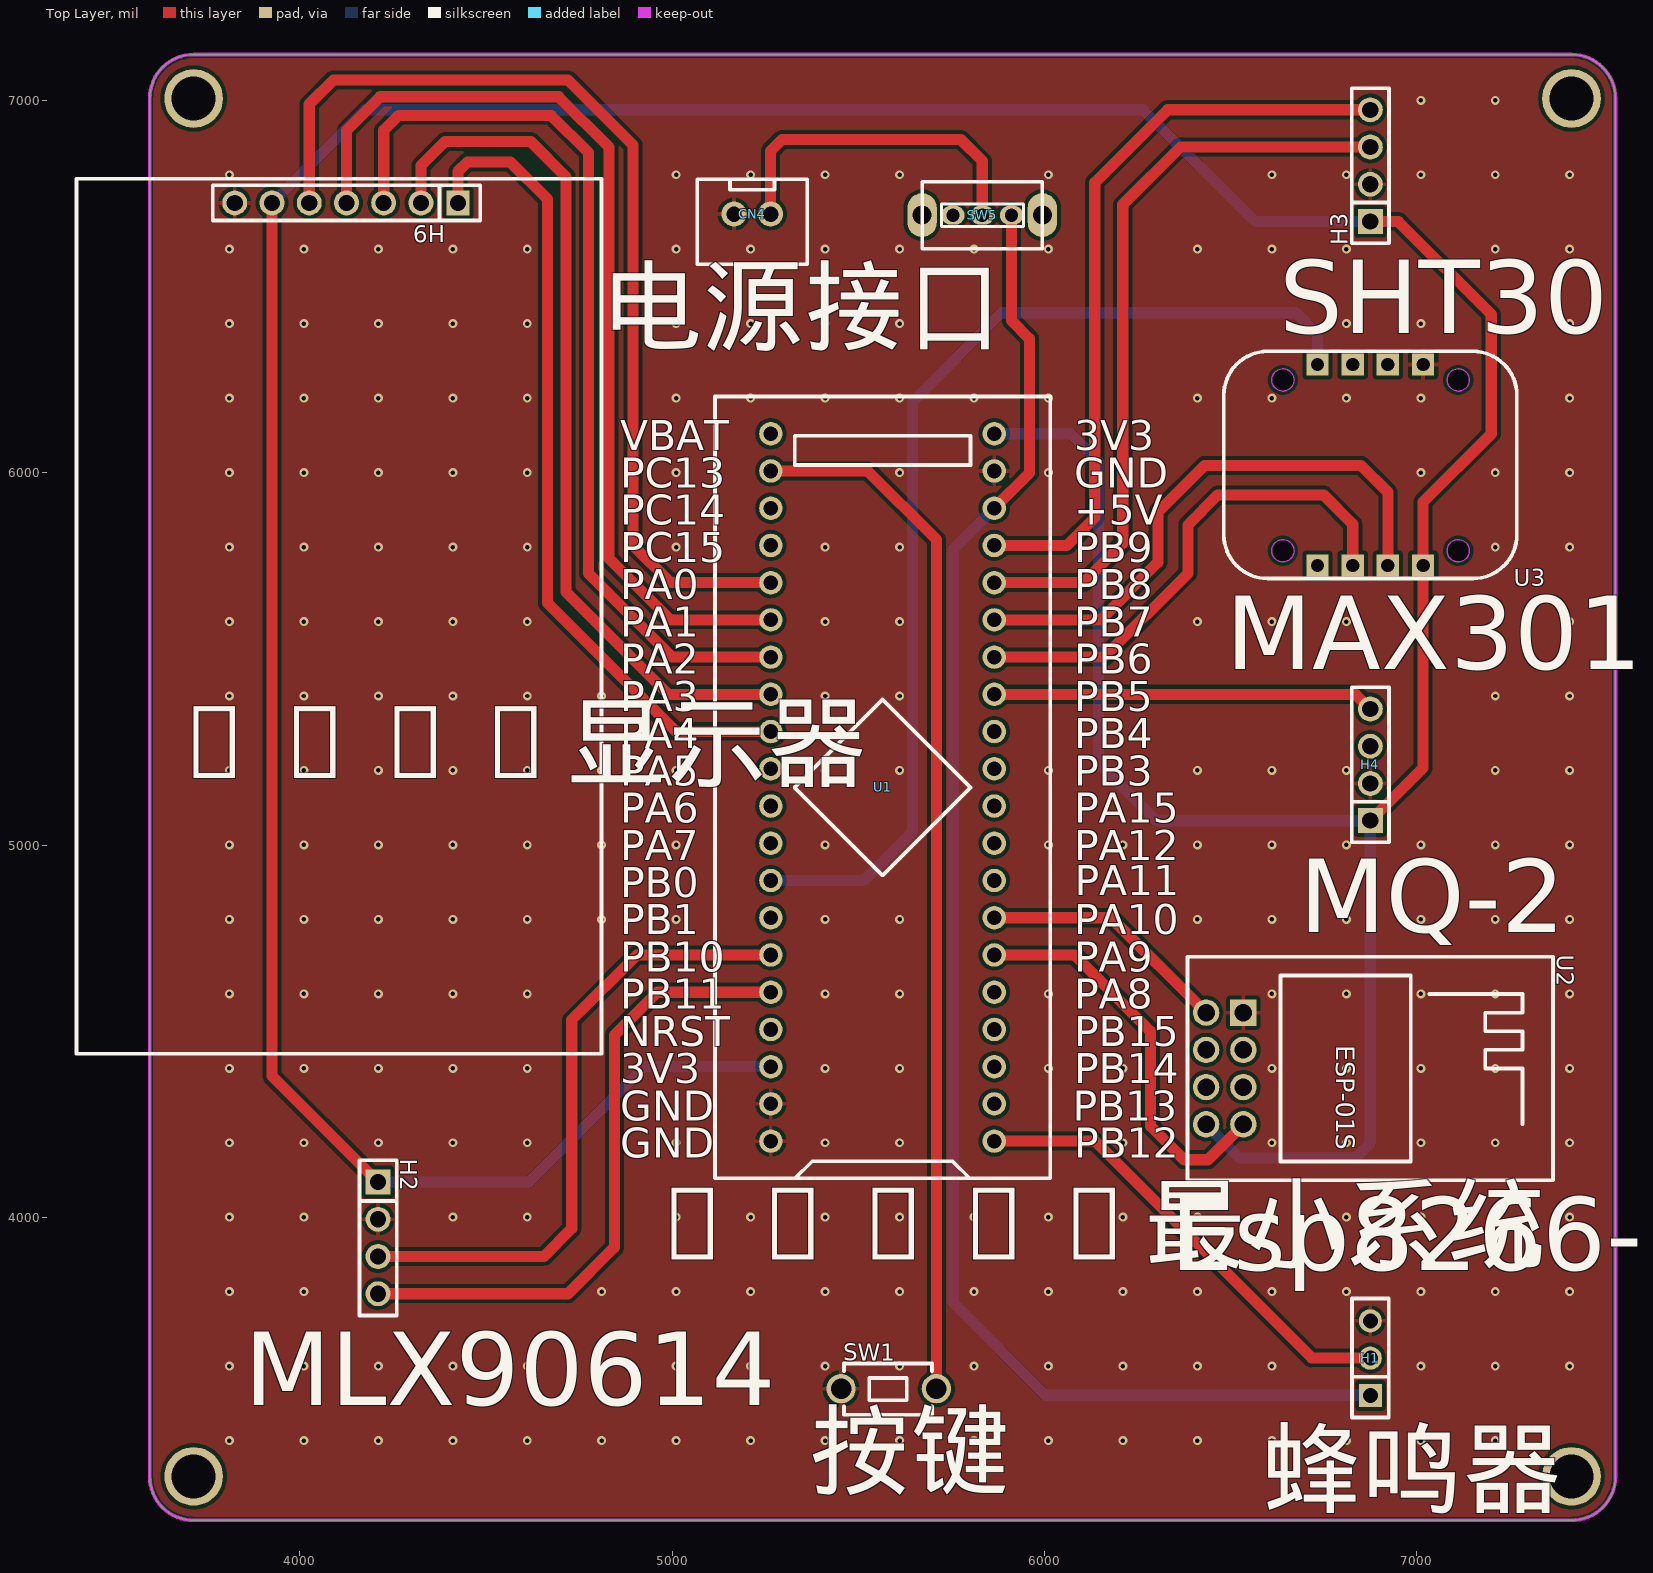
[diagram p0: Top Layer view]
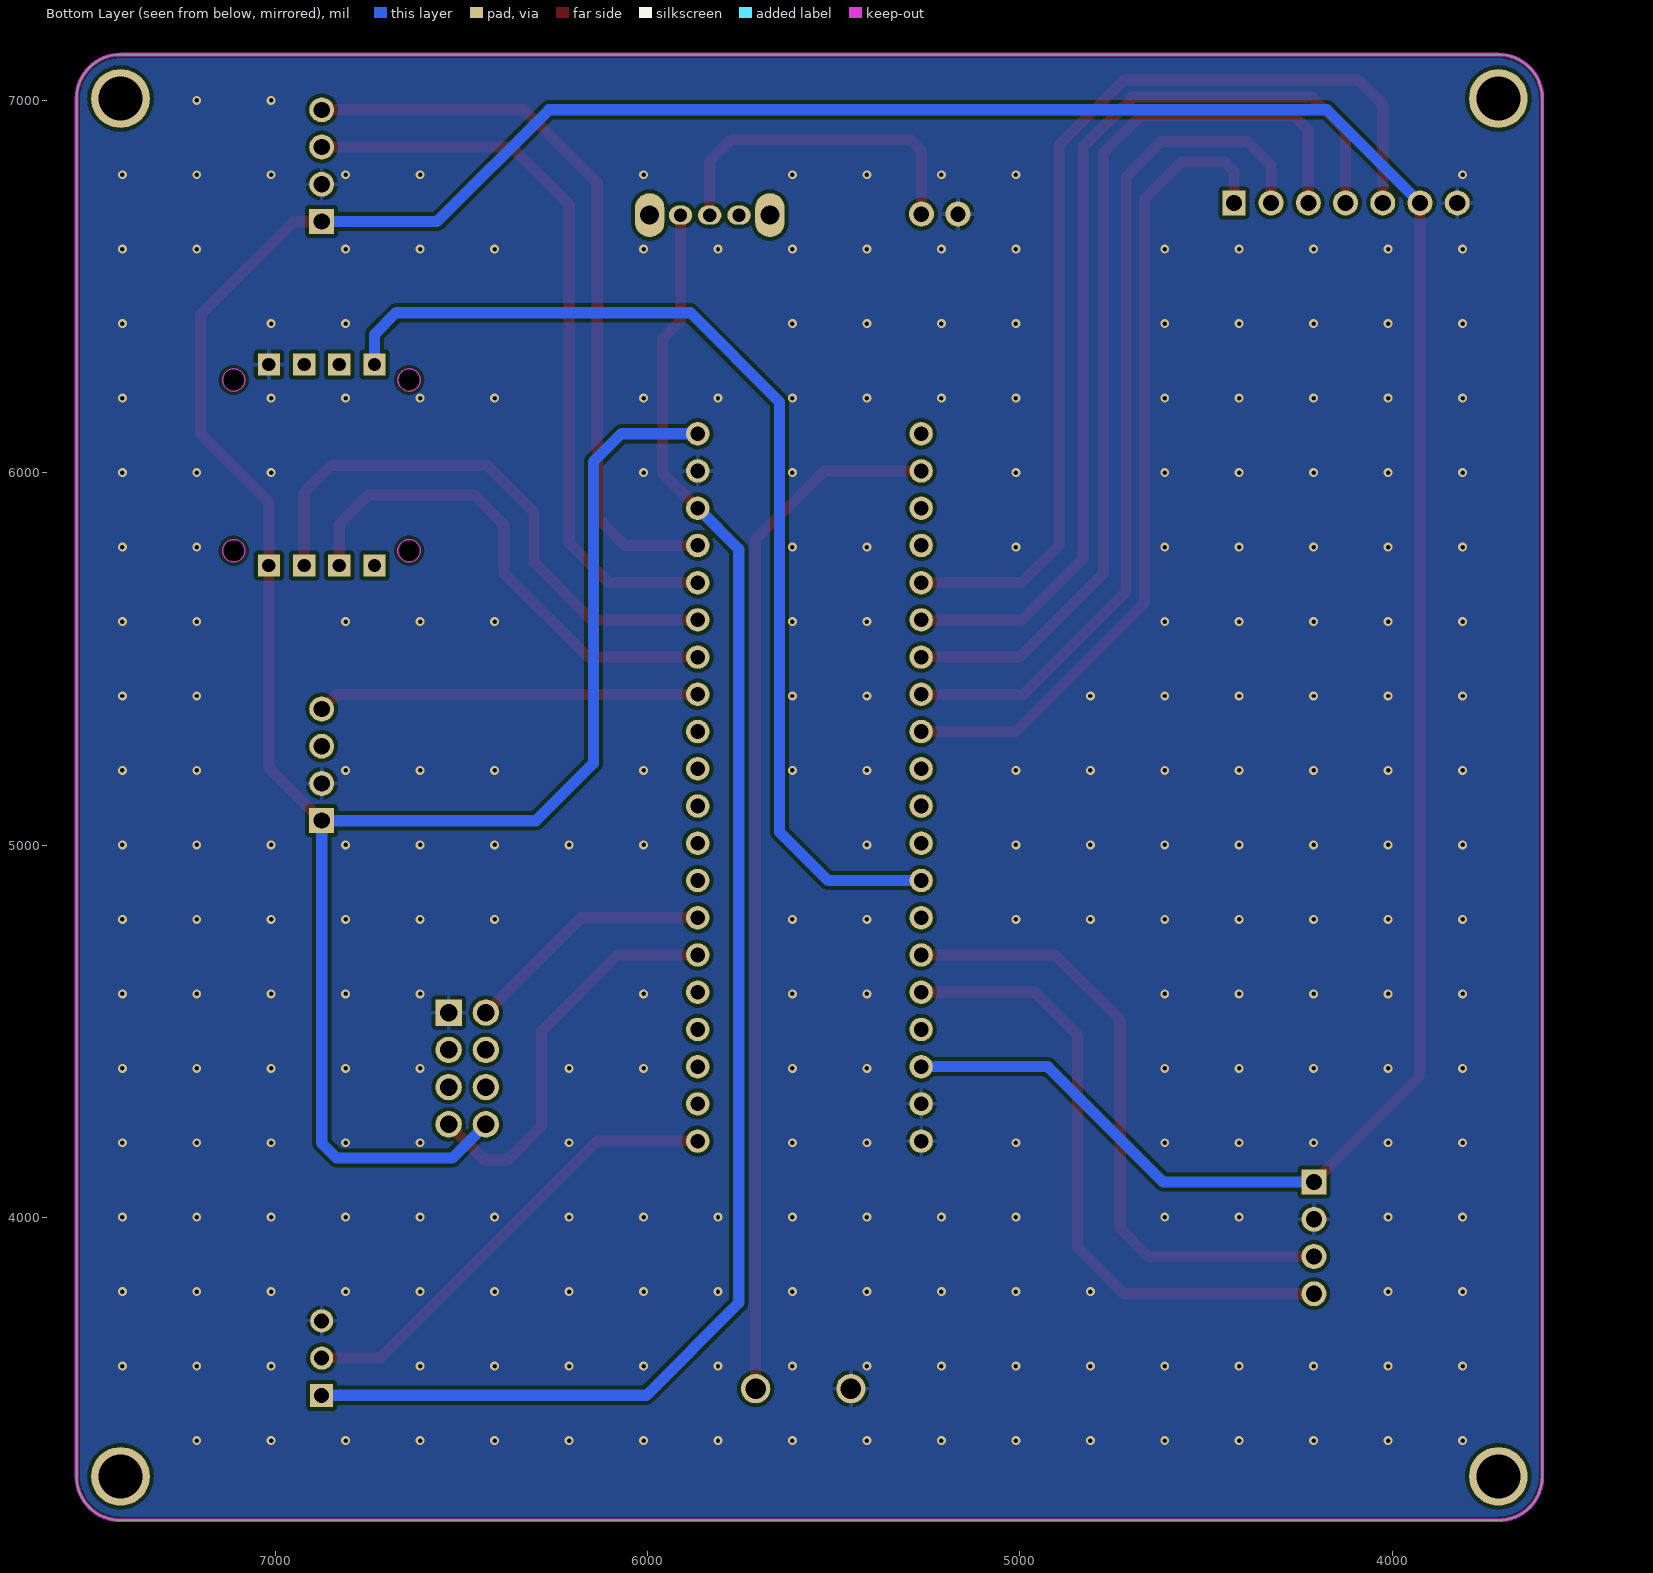
[diagram p1: Bottom Layer view, seen from below]
# Altium PCB MISC52061.pcbdoc
Units mil, origin at the board's own origin, x right, y up, seen from the top; angles counter-clockwise.
Board outline 3937.01 x 3937.01 mil, 2 copper layers (Top Layer, Bottom Layer), stack 62.206 mil thick; 11 components, 38 nets, 91 pads, 256 vias.

## Layer stack, top to bottom
Top Solder Mask Layer: solder mask 0.394, Dk 3.3
Top Layer: signal copper 1.379
Dielectric1: surface 59.449, FR4, Dk 4.5
Bottom Layer: signal copper 1.378
Bottom Solder Mask Layer: solder mask 0.394, Dk 3.3

## Board outline
3714.61,7123.5 ccw(c3714.61,7005.39) 3596.5,7005.39 3596.5,3304.61 ccw(c3714.61,3304.61) 3714.61,3186.5 7415.39,3186.5 ccw(c7415.39,3304.61) 7533.5,3304.61 7533.5,7005.39 ccw(c7415.39,7005.39) 7415.39,7123.5 3714.61,7123.5

## Design rules (kind name [scope] priority, off if disabled: settings)
BoardOutlineClearance copperThickness2oz_1 [All] p2 off: genericclearance=7.99 ignorepadtopadclearanceinfootprint=FALSE except(0: Arc-SplitContinuation Track-SplitContinuation SMDPad-SplitContinuation THPad-SplitContinuation Via-SplitContinuation Fill-SplitContinuation Region-SplitContinuation Poly-SplitContinuation Text-SplitContinuation Hole-SplitContinuation; 5.98: Arc-CutoutEdge Track-CutoutEdge SMDPad-CutoutEdge THPad-CutoutEdge Via-CutoutEdge Text-CutoutEdge; 6.9: Hole-OutlineEdge Hole-CutoutEdge; 10: Poly-OutlineEdge Poly-CutoutEdge; 11.81: Arc-OutlineEdge Track-OutlineEdge SMDPad-OutlineEdge THPad-OutlineEdge Via-OutlineEdge Fill-OutlineEdge Region-OutlineEdge Text-OutlineEdge Fill-CutoutEdge Region-CutoutEdge)
BoardOutlineClearance Plane_innerPlane_1 [All] p4 off: genericclearance=4.02 ignorepadtopadclearanceinfootprint=FALSE except(0: Arc-SplitContinuation Track-SplitContinuation SMDPad-SplitContinuation THPad-SplitContinuation Via-SplitContinuation Fill-SplitContinuation Region-SplitContinuation Poly-SplitContinuation Text-SplitContinuation Hole-SplitContinuation; 5.98: Arc-CutoutEdge Track-CutoutEdge SMDPad-CutoutEdge THPad-CutoutEdge Via-CutoutEdge Text-CutoutEdge; 6.9: Hole-OutlineEdge Hole-CutoutEdge; 10: Poly-OutlineEdge Poly-CutoutEdge; 11.81: Arc-OutlineEdge Track-OutlineEdge SMDPad-OutlineEdge THPad-OutlineEdge Via-OutlineEdge Fill-OutlineEdge Region-OutlineEdge Text-OutlineEdge Fill-CutoutEdge Region-CutoutEdge)
BoardOutlineClearance Copper_copperRegion_1 [All] p6 off: genericclearance=4.02 ignorepadtopadclearanceinfootprint=FALSE except(0: Arc-SplitContinuation Track-SplitContinuation SMDPad-SplitContinuation THPad-SplitContinuation Via-SplitContinuation Fill-SplitContinuation Region-SplitContinuation Poly-SplitContinuation Text-SplitContinuation Hole-SplitContinuation; 5.98: Arc-CutoutEdge Track-CutoutEdge SMDPad-CutoutEdge THPad-CutoutEdge Via-CutoutEdge Text-CutoutEdge; 6.9: Hole-OutlineEdge Hole-CutoutEdge; 10: Poly-OutlineEdge Poly-CutoutEdge; 11.81: Arc-OutlineEdge Track-OutlineEdge SMDPad-OutlineEdge THPad-OutlineEdge Via-OutlineEdge Fill-OutlineEdge Region-OutlineEdge Text-OutlineEdge Fill-CutoutEdge Region-CutoutEdge)
BoardOutlineClearance Copper_copperRegion_copperThickness1oz_1 [All] p8 off: genericclearance=4.02 ignorepadtopadclearanceinfootprint=FALSE except(0: Arc-SplitContinuation Track-SplitContinuation SMDPad-SplitContinuation THPad-SplitContinuation Via-SplitContinuation Fill-SplitContinuation Region-SplitContinuation Poly-SplitContinuation Text-SplitContinuation Hole-SplitContinuation; 5.98: Arc-CutoutEdge Track-CutoutEdge SMDPad-CutoutEdge THPad-CutoutEdge Via-CutoutEdge Text-CutoutEdge; 6.9: Hole-OutlineEdge Hole-CutoutEdge; 10: Poly-OutlineEdge Poly-CutoutEdge; 11.81: Arc-OutlineEdge Track-OutlineEdge SMDPad-OutlineEdge THPad-OutlineEdge Via-OutlineEdge Fill-OutlineEdge Region-OutlineEdge Text-OutlineEdge Fill-CutoutEdge Region-CutoutEdge)
BoardOutlineClearance Copper_copperRegion_Copper_copperRegion_1 [All] p10 off: genericclearance=4.02 ignorepadtopadclearanceinfootprint=FALSE except(0: Arc-SplitContinuation Track-SplitContinuation SMDPad-SplitContinuation THPad-SplitContinuation Via-SplitContinuation Fill-SplitContinuation Region-SplitContinuation Poly-SplitContinuation Text-SplitContinuation Hole-SplitContinuation; 5.98: Arc-CutoutEdge Track-CutoutEdge SMDPad-CutoutEdge THPad-CutoutEdge Via-CutoutEdge Text-CutoutEdge; 6.9: Hole-OutlineEdge Hole-CutoutEdge; 10: Poly-OutlineEdge Poly-CutoutEdge; 11.81: Arc-OutlineEdge Track-OutlineEdge SMDPad-OutlineEdge THPad-OutlineEdge Via-OutlineEdge Fill-OutlineEdge Region-OutlineEdge Text-OutlineEdge Fill-CutoutEdge Region-CutoutEdge)
BoardOutlineClearance copperThickness1oz_1 [All] p12: genericclearance=4.02 ignorepadtopadclearanceinfootprint=FALSE except(0: Arc-SplitContinuation Track-SplitContinuation SMDPad-SplitContinuation THPad-SplitContinuation Via-SplitContinuation Fill-SplitContinuation Region-SplitContinuation Poly-SplitContinuation Text-SplitContinuation Hole-SplitContinuation; 5.98: Arc-CutoutEdge Track-CutoutEdge SMDPad-CutoutEdge THPad-CutoutEdge Via-CutoutEdge Text-CutoutEdge; 6.9: Hole-OutlineEdge Hole-CutoutEdge; 10: Poly-OutlineEdge Poly-CutoutEdge; 11.81: Arc-OutlineEdge Track-OutlineEdge SMDPad-OutlineEdge THPad-OutlineEdge Via-OutlineEdge Fill-OutlineEdge Region-OutlineEdge Text-OutlineEdge Fill-CutoutEdge Region-CutoutEdge)
Clearance copperThickness2oz [All] p1 off: gap=7.99 ignorepadtopadclearanceinfootprint=FALSE except(5.98: SMDPad-Track SMDPad-SMDPad THPad-Track SMDPad-THPad THPad-THPad Track-Via SMDPad-Via THPad-Via Via-Via Fill-SMDPad Region-SMDPad Fill-THPad Region-THPad Fill-Via Region-Via Fill-Fill Fill-Region Region-Region Arc-Track Arc-SMDPad Arc-THPad Arc-Via Fill-Arc Region-Arc Arc-Arc Text-Track SMDPad-Text Text-THPad Text-Via Fill-Text Region-Text Arc-Text Text-Text; 6.9: Hole-Track Hole-SMDPad Hole-THPad Hole-Via Fill-Hole Region-Hole Hole-Arc Hole-Text; 10: Poly-Track Poly-SMDPad Poly-THPad Poly-Via Poly-Fill Poly-Region Poly-Poly Poly-Arc Poly-Text Poly-Hole; 11.81: Fill-Track Region-Track)
Clearance Plane_innerPlane [All] p3 off: gap=4.02 ignorepadtopadclearanceinfootprint=FALSE except(5.98: SMDPad-Track SMDPad-SMDPad THPad-Track SMDPad-THPad THPad-THPad Track-Via SMDPad-Via THPad-Via Via-Via Fill-SMDPad Region-SMDPad Fill-THPad Region-THPad Fill-Via Region-Via Fill-Fill Fill-Region Region-Region Arc-Track Arc-SMDPad Arc-THPad Arc-Via Fill-Arc Region-Arc Arc-Arc Text-Track SMDPad-Text Text-THPad Text-Via Fill-Text Region-Text Arc-Text Text-Text; 6.9: Hole-Track Hole-SMDPad Hole-THPad Hole-Via Fill-Hole Region-Hole Hole-Arc Hole-Text; 10: Poly-Track Poly-SMDPad Poly-THPad Poly-Via Poly-Fill Poly-Region Poly-Poly Poly-Arc Poly-Text Poly-Hole; 11.81: Fill-Track Region-Track)
Clearance Copper_copperRegion [All] p5 off: gap=4.02 ignorepadtopadclearanceinfootprint=FALSE except(5.98: SMDPad-Track SMDPad-SMDPad THPad-Track SMDPad-THPad THPad-THPad Track-Via SMDPad-Via THPad-Via Via-Via Fill-SMDPad Region-SMDPad Fill-THPad Region-THPad Fill-Via Region-Via Fill-Fill Fill-Region Region-Region Arc-Track Arc-SMDPad Arc-THPad Arc-Via Fill-Arc Region-Arc Arc-Arc Text-Track SMDPad-Text Text-THPad Text-Via Fill-Text Region-Text Arc-Text Text-Text; 6.9: Hole-Track Hole-SMDPad Hole-THPad Hole-Via Fill-Hole Region-Hole Hole-Arc Hole-Text; 10: Poly-Track Poly-SMDPad Poly-THPad Poly-Via Poly-Fill Poly-Region Poly-Poly Poly-Arc Poly-Text Poly-Hole; 11.81: Fill-Track Region-Track)
Clearance Copper_copperRegion_copperThickness1oz [All] p7 off: gap=4.02 ignorepadtopadclearanceinfootprint=FALSE except(5.98: SMDPad-Track SMDPad-SMDPad THPad-Track SMDPad-THPad THPad-THPad Track-Via SMDPad-Via THPad-Via Via-Via Fill-SMDPad Region-SMDPad Fill-THPad Region-THPad Fill-Via Region-Via Fill-Fill Fill-Region Region-Region Arc-Track Arc-SMDPad Arc-THPad Arc-Via Fill-Arc Region-Arc Arc-Arc Text-Track SMDPad-Text Text-THPad Text-Via Fill-Text Region-Text Arc-Text Text-Text; 6.9: Hole-Track Hole-SMDPad Hole-THPad Hole-Via Fill-Hole Region-Hole Hole-Arc Hole-Text; 10: Poly-Track Poly-SMDPad Poly-THPad Poly-Via Poly-Fill Poly-Region Poly-Poly Poly-Arc Poly-Text Poly-Hole; 11.81: Fill-Track Region-Track)
Clearance Copper_copperRegion_Copper_copperRegion [All] p9 off: gap=4.02 ignorepadtopadclearanceinfootprint=FALSE except(5.98: SMDPad-Track SMDPad-SMDPad THPad-Track SMDPad-THPad THPad-THPad Track-Via SMDPad-Via THPad-Via Via-Via Fill-SMDPad Region-SMDPad Fill-THPad Region-THPad Fill-Via Region-Via Fill-Fill Fill-Region Region-Region Arc-Track Arc-SMDPad Arc-THPad Arc-Via Fill-Arc Region-Arc Arc-Arc Text-Track SMDPad-Text Text-THPad Text-Via Fill-Text Region-Text Arc-Text Text-Text; 6.9: Hole-Track Hole-SMDPad Hole-THPad Hole-Via Fill-Hole Region-Hole Hole-Arc Hole-Text; 10: Poly-Track Poly-SMDPad Poly-THPad Poly-Via Poly-Fill Poly-Region Poly-Poly Poly-Arc Poly-Text Poly-Hole; 11.81: Fill-Track Region-Track)
Clearance copperThickness1oz [All] p11: gap=4.02 ignorepadtopadclearanceinfootprint=FALSE except(5.98: SMDPad-Track SMDPad-SMDPad THPad-Track SMDPad-THPad THPad-THPad Track-Via SMDPad-Via THPad-Via Via-Via Fill-SMDPad Region-SMDPad Fill-THPad Region-THPad Fill-Via Region-Via Fill-Fill Fill-Region Region-Region Arc-Track Arc-SMDPad Arc-THPad Arc-Via Fill-Arc Region-Arc Arc-Arc Text-Track SMDPad-Text Text-THPad Text-Via Fill-Text Region-Text Arc-Text Text-Text; 6.9: Hole-Track Hole-SMDPad Hole-THPad Hole-Via Fill-Hole Region-Hole Hole-Arc Hole-Text; 10: Poly-Track Poly-SMDPad Poly-THPad Poly-Via Poly-Fill Poly-Region Poly-Poly Poly-Arc Poly-Text Poly-Hole; 11.81: Fill-Track Region-Track)
DiffPairsRouting differentialPair [All] p1: maxlimit=6 minlimit=6 mostfreqgap=6 toplayer_minwidth=5 toplayer_prefwidth=10 toplayer_maxwidth=100 toplayer_mingap=6 toplayer_prefgap=6 toplayer_maxgap=6 bottomlayer_minwidth=5 bottomlayer_prefwidth=10 bottomlayer_maxwidth=100 bottomlayer_mingap=6 bottomlayer_prefgap=6 bottomlayer_maxgap=6 maxuncoupledlength=10
HoleToHoleClearance otherClearance [All] p1: gap=11.81 allowstackedmicrovias=TRUE
Length netLength [All] p1: minlimit=0 maxlimit=0
PasteMaskExpansion pasteMaskExpansion [All] p1: expansion=0
PlaneConnect innerPlane [All] p1: planeconnectstyle=Relief reliefexpansion=20 reliefentries=4 reliefconductorwidth=10 reliefairgap=10
PolygonConnect copperRegion_copperThickness1oz [All] p1 off: connectstyle=Relief reliefconductorwidth=10 reliefentries=4 polygonreliefangle="90 Angle" airgapwidth=10 via.connectstyle=Relief via.reliefconductorwidth=10 via.reliefentries=4 via.polygonreliefangle="90 Angle" via.airgapwidth=10
PolygonConnect copperRegion_Copper_copperRegion [All] p2 off: connectstyle=Relief reliefconductorwidth=10 reliefentries=4 polygonreliefangle="90 Angle" airgapwidth=10 via.connectstyle=Relief via.reliefconductorwidth=10 via.reliefentries=4 via.polygonreliefangle="90 Angle" via.airgapwidth=10
PolygonConnect copperRegion [All] p3: connectstyle=Relief reliefconductorwidth=10 reliefentries=4 polygonreliefangle="90 Angle" airgapwidth=10 via.connectstyle=Relief via.reliefconductorwidth=10 via.reliefentries=4 via.polygonreliefangle="90 Angle" via.airgapwidth=10
RoutingVias viaSize [All] p1: holewidth=12.01 width=24.02 viastyle="Through Hole" minholewidth=11.81 minwidth=19.68 maxholewidth=248.03 maxwidth=393.7
SolderMaskExpansion solderMaskExpansion [IsVia] p1: expansion=-1000 istentingtop=TRUE
SolderMaskExpansion solderMaskExpansion [All] p2: expansion=2 istentingtop=FALSE
Width copperThickness2oz_2 [All] p1 off: maxlimit=100 minlimit=8 preferedwidth=10
Width copperThickness1oz_2 [All] p2: maxlimit=100 minlimit=5 preferedwidth=10

## Components (designator, comment, footprint, x,y, rotation, side; value= is the part's Value field where it differs from the comment)
CN4 "XH2.54*2P_直插" CONN-TH_2P-P2.50-XH2.54-2P 5215,6695 r0 top
H1 "" HDR-TH_3P-P2.54-V-F 6875,3622.19 r90 top
H2 "" HDR-TH_4P-P2.54-V-F 4210,3945 r270 top
H3 "" HDR-TH_4P-P2.54-V-F 6875,6825 r90 top
H4 "" HDR-TH_4P-P2.54-V-F 6875,5215.69 r90 top
H9 "" HDR-TH_7P-P2.54-V-F 4125,6725 r180 top
SW1 "" Key_TH_3.5x6x4.3 5575,3540 r0 top
SW5 "" 拨动开关 5837.9,6692.05 r180 top
U1 "STM32F103C8T6-Card" CONN-TH_L53.3-W22.9_STM32F103C8T6-CARD 5565,5155 r90 top
U2 "ESP-01S" WIFIM-TH_ESP-01S 6484,4400.1 r270 top
U3 "MAX30102" MAX30102 7268.7,5715.97 r180 top

## Footprints (in the part's own frame and the unit in brackets; to place one, negate y for a bottom-side part, rotate by r counter-clockwise, add the part's x,y. Pads: shape width x height; smd on the part's side, far side on the other; paste and mask are expansions set on the pad)
CONN-TH_2P-P2.50-XH2.54-2P [mm]
  round 1.7 hole 1.05 paste+0 mask+0.05: 1(1.25,0) 2(-1.25,0)
  silkscreen extent -3.75,-3.42 3.75,2.37
CONN-TH_L53.3-W22.9_STM32F103C8T6-CARD [mm]
  round 1.6 hole 1: 1(-24.13,-7.62) 2(-21.59,-7.62) 3(-19.05,-7.62) 4(-16.51,-7.62) 5(-13.97,-7.62) 6(-11.43,-7.62) 7(-8.89,-7.62) 8(-6.35,-7.62) 9(-3.81,-7.62) 10(-1.27,-7.62) 11(1.27,-7.62) 12(3.81,-7.62) 13(6.35,-7.62) 14(8.89,-7.62) 15(11.43,-7.62) 16(13.97,-7.62) 17(16.51,-7.62) 18(19.05,-7.62) 19(21.59,-7.62) 20(24.13,-7.62) 21(24.13,7.62) 22(21.59,7.62) 23(19.05,7.62) 24(16.51,7.62) 25(13.97,7.62) 26(11.43,7.62) 27(8.89,7.62) 28(6.35,7.62) 29(3.81,7.62) 30(1.27,7.62) 31(-1.27,7.62) 32(-3.81,7.62) 33(-6.35,7.62) 34(-8.89,7.62) 35(-11.43,7.62) 36(-13.97,7.62) 37(-16.51,7.62) 38(-19.05,7.62) 39(-21.59,7.62) 40(-24.13,7.62)
  silkscreen extent -26.67,-11.43 26.67,11.43
HDR-TH_3P-P2.54-V-F [mil]
  rect 62x62 hole 40.16: 1(-100,0)
  round 62 hole 40.16: 2(0,0) 3(100,0)
  silkscreen extent -160,-49 160,49
HDR-TH_4P-P2.54-V-F [mm]
  rect 1.7x1.7 hole 1.1: 1(-3.81,0)
  round 1.7 hole 1.1: 2(-1.27,0) 3(1.27,0) 4(3.81,0)
  silkscreen extent -5.29,-1.27 5.29,1.27
HDR-TH_7P-P2.54-V-F [mm]
  rect 1.575x1.7 hole 1.1: 1(-7.62,0)
  round 1.7 hole 1.1: 2(-5.08,0) 3(-2.54,0) 4(0,0) 5(2.54,0) 6(5.08,0) 7(7.62,0)
  silkscreen extent -9.13,-1.2 9.13,1.2
Key_TH_3.5x6x4.3 [mil]
  round 78.7 hole 55.1 paste+0 mask+2: A(-121.44,0) B(134.46,0)
  silkscreen extent -114,-70 123,68
MAX30102 [mil]
  rect 60x60 hole 36: 1(251.97,-35) 2(346.46,-35) 3(440.94,-35) 4(535.43,-35) 5(251.97,-575) 6(346.46,-575) 7(440.94,-575) 8(535.43,-575)
  Board Outline Layer circle w0.1: c157.48,-74.8 r30
  Board Outline Layer circle w0.1: c157.48,-533.46 r30
  Board Outline Layer circle w0.1: c628.5,-74.8 r30
  Board Outline Layer circle w0.1: c628.5,-533.46 r30
  Board Outline Layer region: 127.48,-74.8 130.45,-61.79 138.78,-51.35 150.8,-45.56 164.16,-45.56 176.18,-51.35 184.51,-61.79 187.48,-74.8 187.48,-74.8 184.51,-87.82 176.18,-98.26 164.16,-104.05 150.8,-104.05 138.78,-98.26 130.45,-87.82 127.48,-74.8
  Board Outline Layer region: 127.48,-74.8 127.85,-70.11 128.95,-65.53 130.75,-61.18 133.21,-57.17 136.27,-53.59 139.85,-50.53 143.86,-48.07 148.21,-46.27 152.79,-45.17 157.48,-44.8 162.17,-45.17 166.75,-46.27 171.1,-48.07 175.11,-50.53 178.69,-53.59 181.75,-57.17 184.21,-61.18 186.01,-65.53 187.11,-70.11 187.48,-74.8 187.11,-79.5 186.01,-84.07 184.21,-88.42 181.75,-92.44 178.69,-96.02 175.11,-99.07 171.1,-101.53 166.75,-103.33 162.17,-104.43 157.48,-104.8 152.79,-104.43 148.21,-103.33 143.86,-101.53 139.85,-99.07 136.27,-96.02 133.21,-92.44 130.75,-88.42 128.95,-84.07 127.85,-79.5
  Board Outline Layer region: 127.48,-533.46 130.45,-520.45 138.78,-510.01 150.8,-504.22 164.16,-504.22 176.18,-510.01 184.51,-520.45 187.48,-533.46 187.48,-533.46 184.51,-546.48 176.18,-556.92 164.16,-562.71 150.8,-562.71 138.78,-556.92 130.45,-546.48 127.48,-533.46
  Board Outline Layer region: 127.48,-533.46 127.85,-528.77 128.95,-524.19 130.75,-519.84 133.21,-515.83 136.27,-512.25 139.85,-509.19 143.86,-506.73 148.21,-504.93 152.79,-503.83 157.48,-503.46 162.17,-503.83 166.75,-504.93 171.1,-506.73 175.11,-509.19 178.69,-512.25 181.75,-515.83 184.21,-519.84 186.01,-524.19 187.11,-528.77 187.48,-533.46 187.11,-538.16 186.01,-542.74 184.21,-547.08 181.75,-551.1 178.69,-554.68 175.11,-557.74 171.1,-560.19 166.75,-562 162.17,-563.1 157.48,-563.46 152.79,-563.1 148.21,-562 143.86,-560.19 139.85,-557.74 136.27,-554.68 133.21,-551.1 130.75,-547.08 128.95,-542.74 127.85,-538.16
  Board Outline Layer region: 598.5,-74.8 601.47,-61.79 609.8,-51.35 621.83,-45.56 635.18,-45.56 647.21,-51.35 655.53,-61.79 658.5,-74.8 658.5,-74.8 655.53,-87.82 647.21,-98.26 635.18,-104.05 621.83,-104.05 609.8,-98.26 601.47,-87.82 598.5,-74.8
  Board Outline Layer region: 598.5,-74.8 598.87,-70.11 599.97,-65.53 601.77,-61.18 604.23,-57.17 607.29,-53.59 610.87,-50.53 614.88,-48.07 619.23,-46.27 623.81,-45.17 628.5,-44.8 633.2,-45.17 637.77,-46.27 642.12,-48.07 646.14,-50.53 649.72,-53.59 652.77,-57.17 655.23,-61.18 657.04,-65.53 658.13,-70.11 658.5,-74.8 658.13,-79.5 657.04,-84.07 655.23,-88.42 652.77,-92.44 649.72,-96.02 646.14,-99.07 642.12,-101.53 637.77,-103.33 633.2,-104.43 628.5,-104.8 623.81,-104.43 619.23,-103.33 614.88,-101.53 610.87,-99.07 607.29,-96.02 604.23,-92.44 601.77,-88.42 599.97,-84.07 598.87,-79.5
  Board Outline Layer region: 598.5,-533.46 601.47,-520.45 609.8,-510.01 621.83,-504.22 635.18,-504.22 647.21,-510.01 655.53,-520.45 658.5,-533.46 658.5,-533.46 655.53,-546.48 647.21,-556.92 635.18,-562.71 621.83,-562.71 609.8,-556.92 601.47,-546.48 598.5,-533.46
  Board Outline Layer region: 598.5,-533.46 598.87,-528.77 599.97,-524.19 601.77,-519.84 604.23,-515.83 607.29,-512.25 610.87,-509.19 614.88,-506.73 619.23,-504.93 623.81,-503.83 628.5,-503.46 633.2,-503.83 637.77,-504.93 642.12,-506.73 646.14,-509.19 649.72,-512.25 652.77,-515.83 655.23,-519.84 657.04,-524.19 658.13,-528.77 658.5,-533.46 658.13,-538.16 657.04,-542.74 655.23,-547.08 652.77,-551.1 649.72,-554.68 646.14,-557.74 642.12,-560.19 637.77,-562 633.2,-563.1 628.5,-563.46 623.81,-563.1 619.23,-562 614.88,-560.19 610.87,-557.74 607.29,-554.68 604.23,-551.1 601.77,-547.08 599.97,-542.74 598.87,-538.16
  Multi-Layer board cut-out: 127.48,-74.8 130.45,-61.79 138.78,-51.35 150.8,-45.56 164.16,-45.56 176.18,-51.35 184.51,-61.79 187.48,-74.8 187.48,-74.8 184.51,-87.82 176.18,-98.26 164.16,-104.05 150.8,-104.05 138.78,-98.26 130.45,-87.82 127.48,-74.8
  Multi-Layer board cut-out: 127.48,-533.46 130.45,-520.45 138.78,-510.01 150.8,-504.22 164.16,-504.22 176.18,-510.01 184.51,-520.45 187.48,-533.46 187.48,-533.46 184.51,-546.48 176.18,-556.92 164.16,-562.71 150.8,-562.71 138.78,-556.92 130.45,-546.48 127.48,-533.46
  Multi-Layer board cut-out: 598.5,-74.8 601.47,-61.79 609.8,-51.35 621.83,-45.56 635.18,-45.56 647.21,-51.35 655.53,-61.79 658.5,-74.8 658.5,-74.8 655.53,-87.82 647.21,-98.26 635.18,-104.05 621.83,-104.05 609.8,-98.26 601.47,-87.82 598.5,-74.8
  Multi-Layer board cut-out: 598.5,-533.46 601.47,-520.45 609.8,-510.01 621.83,-504.22 635.18,-504.22 647.21,-510.01 655.53,-520.45 658.5,-533.46 658.5,-533.46 655.53,-546.48 647.21,-556.92 635.18,-562.71 621.83,-562.71 609.8,-556.92 601.47,-546.48 598.5,-533.46
  silkscreen extent 0,-610 787,0
WIFIM-TH_ESP-01S [mm]
  rect 1.8x1.8 hole 1.2: 1(-3.81,1.27)
  round 1.8 hole 1.2: 2(-1.27,1.27) 3(1.27,1.27) 4(3.81,1.27) 5(3.81,-1.27) 6(1.27,-1.27) 7(-1.27,-1.27) 8(-3.81,-1.27)
  silkscreen extent -7.62,-2.54 7.62,22.4
拨动开关 [mil]
  oval 63x51.2 hole 35.4 paste+0 mask+2: 1(-73.4,0) 2(5,0) 3(84,0)
  oval 78.7x118.1 hole 51.2 paste+0 mask+2: 4(166.7,0) 5(-156.1,0)
  silkscreen extent -156,-90 167,90

## Free pads (board coordinates)
  round 157.48 hole 118.11: 1(3714.61,7005.39) 1(3714.61,3304.61) 1(7415.39,7005.39) 1(7415.39,3304.61)

## Via types
v1: diameter 24.02, hole 12, Top Layer to Bottom Layer, 256 vias

## Nets (pads, with @x,y where several pads share a name; then routed paths per layer and width w, separated by ;. In a path a pad name is that pad's centre, name@x,y a point inside that pad or via, vN(x,y) a via of type N, cw(c..) or ccw(c..) an arc to the next point about the centre after c; other vN are vias at no path point)
$1N17118: CN4.1 SW5.2 | length 919.7
  Top Layer w30: CN4.1 5264.22,6864.22 5295,6895 5775,6895 5832.9,6837.1 SW5.2
+5V: H1.1 SW5.1 U1.18 | length 4249.8
  Top Layer w30: U1.18 5960,6000 5960,6360 5911.3,6408.7 SW5.1
  Bottom Layer w30: U1.18 5755,5795 5755,3770 6002.81,3522.19 H1.1
GND: CN4.2 H1.3 H2.2 H3.2 H4.2 H9.7 SW1.A U1.19 U1.39 U1.40 U2.1 U3.5
  other v1: 3810.6,3400.6 4010.6,3400.6 4210.6,3400.6 4410.6,3400.6 4610.6,3400.6 4810.6,3400.6 5010.6,3400.6 5210.6,3400.6 5410.6,3400.6 5610.6,3400.6 5810.6,3400.6 6010.6,3400.6 6210.6,3400.6 6410.6,3400.6 6610.6,3400.6 6810.6,3400.6 7010.6,3400.6 7210.6,3400.6 3810.6,3600.6 4010.6,3600.6 4210.6,3600.6 4410.6,3600.6 4610.6,3600.6 4810.6,3600.6 5010.6,3600.6 5210.6,3600.6 5410.6,3600.6 5610.6,3600.6 5810.6,3600.6 6010.6,3600.6 6210.6,3600.6 6410.6,3600.6 6610.6,3600.6 7010.6,3600.6 7210.6,3600.6 7410.6,3600.6 3810.6,3800.6 4010.6,3800.6 4810.6,3800.6 5010.6,3800.6 5210.6,3800.6 5410.6,3800.6 5610.6,3800.6 5810.6,3800.6 6010.6,3800.6 6210.6,3800.6 6410.6,3800.6 6610.6,3800.6 6810.6,3800.6 7010.6,3800.6 7210.6,3800.6 7410.6,3800.6 3810.6,4000.6 4010.6,4000.6 4410.6,4000.6 4610.6,4000.6 5010.6,4000.6 5210.6,4000.6 5410.6,4000.6 5610.6,4000.6 5810.6,4000.6 6010.6,4000.6 6210.6,4000.6 6410.6,4000.6 6610.6,4000.6 6810.6,4000.6 7010.6,4000.6 7210.6,4000.6 7410.6,4000.6 3810.6,4200.6 4010.6,4200.6 4210.6,4200.6 4410.6,4200.6 4610.6,4200.6 5010.6,4200.6 5410.6,4200.6 5610.6,4200.6 6210.6,4200.6 6610.6,4200.6 6810.6,4200.6 7010.6,4200.6 7210.6,4200.6 7410.6,4200.6 3810.6,4400.6 4010.6,4400.6 4210.6,4400.6 4410.6,4400.6 4610.6,4400.6 5410.6,4400.6 5610.6,4400.6 6010.6,4400.6 6210.6,4400.6 6610.6,4400.6 6810.6,4400.6 7010.6,4400.6 7210.6,4400.6 7410.6,4400.6 3810.6,4600.6 4010.6,4600.6 4210.6,4600.6 4410.6,4600.6 4610.6,4600.6 5410.6,4600.6 5610.6,4600.6 6010.6,4600.6 6610.6,4600.6 6810.6,4600.6 7010.6,4600.6 7210.6,4600.6 7410.6,4600.6 3810.6,4800.6 4010.6,4800.6 4210.6,4800.6 4410.6,4800.6 4610.6,4800.6 4810.6,4800.6 5010.6,4800.6 5410.6,4800.6 5610.6,4800.6 6410.6,4800.6 6610.6,4800.6 6810.6,4800.6 7010.6,4800.6 7210.6,4800.6 7410.6,4800.6 3810.6,5000.6 4010.6,5000.6 4210.6,5000.6 4410.6,5000.6 4610.6,5000.6 4810.6,5000.6 5010.6,5000.6 5410.6,5000.6 6010.6,5000.6 6210.6,5000.6 6410.6,5000.6 6610.6,5000.6 6810.6,5000.6 7010.6,5000.6 7210.6,5000.6 7410.6,5000.6 3810.6,5200.6 4010.6,5200.6 4210.6,5200.6 4410.6,5200.6 4610.6,5200.6 4810.6,5200.6 5010.6,5200.6 5410.6,5200.6 5610.6,5200.6 6010.6,5200.6 6410.6,5200.6 6610.6,5200.6 6810.6,5200.6 7210.6,5200.6 7410.6,5200.6 3810.6,5400.6 4010.6,5400.6 4210.6,5400.6 4410.6,5400.6 4610.6,5400.6 4810.6,5400.6 5410.6,5400.6 5610.6,5400.6 7210.6,5400.6 7410.6,5400.6 3810.6,5600.6 4010.6,5600.6 4210.6,5600.6 4410.6,5600.6 4610.6,5600.6 5410.6,5600.6 5610.6,5600.6 6410.6,5600.6 6610.6,5600.6 6810.6,5600.6 7210.6,5600.6 7410.6,5600.6 3810.6,5800.6 4010.6,5800.6 4210.6,5800.6 4410.6,5800.6 4610.6,5800.6 5010.6,5800.6 5410.6,5800.6 5610.6,5800.6 7210.6,5800.6 7410.6,5800.6 3810.6,6000.6 4010.6,6000.6 4210.6,6000.6 4410.6,6000.6 4610.6,6000.6 5010.6,6000.6 5610.6,6000.6 6010.6,6000.6 7010.6,6000.6 7210.6,6000.6 7410.6,6000.6 3810.6,6200.6 4010.6,6200.6 4210.6,6200.6 4410.6,6200.6 4610.6,6200.6 5010.6,6200.6 5210.6,6200.6 5410.6,6200.6 5610.6,6200.6 5810.6,6200.6 6010.6,6200.6 6410.6,6200.6 6610.6,6200.6 6810.6,6200.6 7010.6,6200.6 7410.6,6200.6 3810.6,6400.6 4010.6,6400.6 4210.6,6400.6 4410.6,6400.6 4610.6,6400.6 5010.6,6400.6 5210.6,6400.6 5410.6,6400.6 5610.6,6400.6 6810.6,6400.6 7010.6,6400.6 7410.6,6400.6 3810.6,6600.6 4010.6,6600.6 4210.6,6600.6 4410.6,6600.6 4610.6,6600.6 5010.6,6600.6 5210.6,6600.6 5410.6,6600.6 5610.6,6600.6 5810.6,6600.6 6010.6,6600.6 6410.6,6600.6 6610.6,6600.6 6810.6,6600.6 7210.6,6600.6 7410.6,6600.6 3810.6,6800.6 5010.6,6800.6 5210.6,6800.6 5410.6,6800.6 5610.6,6800.6 6010.6,6800.6 6610.6,6800.6 6810.6,6800.6 7010.6,6800.6 7210.6,6800.6 7410.6,6800.6 7010.6,7000.6 7210.6,7000.6
NRST: U1.37
PA0: H9.5 U1.25 | length 2720.8
  Top Layer w30: H9.5 4025,6990 4090,7055 4720,7055 4895,6880 4895,5805 4995,5705 U1.25
PA1: H9.4 U1.26 | length 2601.5
  Top Layer w30: H9.4 4125,6920 4215,7010 4695,7010 4830,6875 4830,5770 4995,5605 U1.26
PA2: H9.3 U1.27 | length 2516.2
  Top Layer w30: H9.3 4225,6920 4265,6960 4675,6960 4775,6860 4775,5730 5000,5505 U1.27
PA3: H9.2 U1.28 | length 2335.2
  Top Layer w30: H9.2 4325,6825 4390,6890 4620,6890 4715,6795 4715,5680 4990,5405 U1.28
PA4: H9.1 U1.29 | length 2204.7
  Top Layer w30: H9.1 4425,6810 4450,6835 4565,6835 4665,6735 4665,5650 5010,5305 U1.29
PA5: U1.30
PA6: U1.31
PA7: U1.32
PA8: U1.5
PA9: U1.6 U2.4 | length 1085.6
  Top Layer w30: U1.6 6080,4705 6285,4500 6285,4245 6375,4155 6438.9,4155 U2.4
PA10: U1.7 U2.8 | length 674.6
  Top Layer w30: U1.7 6179.1,4805 U2.8
PA11: U1.8
PA12: U1.9
PA15: U1.10
PB0: U1.33 U3.8 | length 2881.4
  Bottom Layer w30: U1.33 5515,4905 5645,5035 5645,6190 5885,6430 6675,6430 6733.27,6371.73 U3.8
PB1: U1.34
PB3: U1.11
PB4: U1.12
PB5: H4.4 U1.13 | length 1026.3
  Top Layer w30: U1.13 6835.69,5405 H4.4
PB6: U1.14 U3.3 | length 1362.6
  Top Layer w30: U1.14 6160,5505 6385,5730 6385,5860 6465,5940 6750,5940 6827.76,5862.24 U3.3
PB7: U1.15 U3.2 | length 1534.9
  Top Layer w30: U1.15 6150,5605 6305,5760 6305,5895 6430,6020 6850,6020 6922.24,5947.76 U3.2
PB8: H3.3 U1.16 | length 2027.7
  Top Layer w30: U1.16 6105,5705 6210,5810 6210,6720 6365,6875 H3.3
PB9: H3.4 U1.17 | length 2021.8
  Top Layer w30: U1.17 6060,5805 6135,5880 6135,6780 6330,6975 H3.4
PB10: H2.3 U1.35 | length 1718.6
  Top Layer w30: H2.3 4655,3895 4730,3970 4730,4530 4905,4705 U1.35
PB11: H2.4 U1.36 | length 1724.4
  Top Layer w30: H2.4 4720,3795 4845,3920 4845,4490 4960,4605 U1.36
PB12: H1.2 U1.1 | length 1251.4
  Top Layer w30: U1.1 6135,4205 6717.81,3622.19 H1.2
PB13: U1.2
PB14: U1.3
PB15: U1.4
PC13: SW1.B U1.22 | length 2801.4
  Top Layer w30: U1.22 5525,6005 5709.46,5820.54 SW1.B
PC14: U1.23
PC15: U1.24
VBAT: U1.21
VCC: H2.1 H3.1 H4.1 H9.6 U1.20 U1.38 U2.5 U3.1 | length 12307.3
  Top Layer w30: H9.6 3925,4380 H2.1 ; H4.1 7016.73,5207.42 U3.1 7016.73,5921.73 7200,6105 7200,6425 6950,6675 H3.1
  Bottom Layer w30: H9.6 4175,6975 6265,6975 6565,6675 H3.1 ; H2.1 4615,4095 4925,4405 U1.38 ; U1.20 6070,6105 6145,6030 6145,5220 6299.31,5065.69 H4.1 6875,4200 6835,4160 6524.1,4160 U2.5
pads on no net: H4.3 SW5.3 SW5.4 SW5.5 U2.2 U2.3 U2.6 U2.7 U3.4 U3.6 U3.7

## Polygon pours and split planes (outlines as drawn)
GND on Bottom Layer (solid, remove dead copper, pour order 2): 3525,7245 3525,3080 7700,3080 7700,7245
GND on Top Layer (solid, remove dead copper, pour order 2): 3000,7415 3000,3000 7930,3000 7930,7415

## Keep-outs
Board Outline Layer:
  the board outline again, w10

## Silkscreen, mask and mechanical layers (free items; w line width, h text height)
Top Silkscreen Layer:
  lines w10: 3400,4440 3400,6790 4810,6790 4810,4440 3400,4440
  text "SHT30" at 6629.83,6374.84 h196.85
  text "电源接口" at 4812.87,6351.57 h196.85
  text "VBAT" at 4860.95,6060 h80
  text "3V3" at 6079.16,6060 h80
  text "PC13" at 4860.95,5960 h80
  text "GND" at 6079.16,5960 h80
  text "PC14" at 4860.95,5860 h80
  text "+5V" at 6079.16,5860 h80
  text "PC15" at 4860.95,5760 h80
  text "PB9" at 6079.16,5760 h80
  text "PA0" at 4860.95,5660 h80
  text "PB8" at 6079.16,5660 h80
  text "PA1" at 4860.95,5560 h80
  text "PB7" at 6079.16,5560 h80
  text "MAX30102" at 6486.82,5472.59 h196.85
  text "PA2" at 4860.95,5460 h80
  text "PB6" at 6079.16,5460 h80
  text "PA3" at 4860.95,5360 h80
  text "PB5" at 6079.16,5360 h80
  text "PA4" at 4860.95,5260 h80
  text "PB4" at 6079.16,5260 h80
  text "Oled显示器" at 3635,5180 h196.85
  text "PA5" at 4860.95,5160 h80
  text "PB3" at 6079.16,5160 h80
  text "PA6" at 4860.95,5060 h80
  text "PA15" at 6079.16,5060 h80
  text "PA7" at 4860.95,4960 h80
  text "PA12" at 6079.16,4960 h80
  text "PA11" at 6080.95,4865 h80
  text "PB0" at 4860.95,4860 h80
  text "MQ-2" at 6683.67,4765.53 h196.85
  text "PB1" at 4860.95,4760 h80
  text "PA10" at 6079.16,4760 h80
  text "PB10" at 4860.95,4660 h80
  text "PA9" at 6079.16,4660 h80
  text "PB11" at 4860.95,4560 h80
  text "PA8" at 6079.16,4560 h80
  text "NRST" at 4860.95,4460 h80
  text "PB15" at 6079.16,4460 h80
  text "3V3" at 4860.95,4360 h80
  text "PB14" at 6079.16,4360 h80
  text "GND" at 4860.95,4260 h80
  text "PB13" at 6075.95,4260 h80
  text "GND" at 4860.95,4160 h80
  text "PB12" at 6079.16,4160 h80
  text "STM32最小系统" at 4919.45,3886.57 h196.85
  text "Esp8266-01s" at 6338.14,3857.51 h196.85
  text "MLX90614" at 3850,3495 h196.85
  text "按键" at 5370,3280 h196.85
  text "蜂鸣器" at 6581.81,3230 h196.85